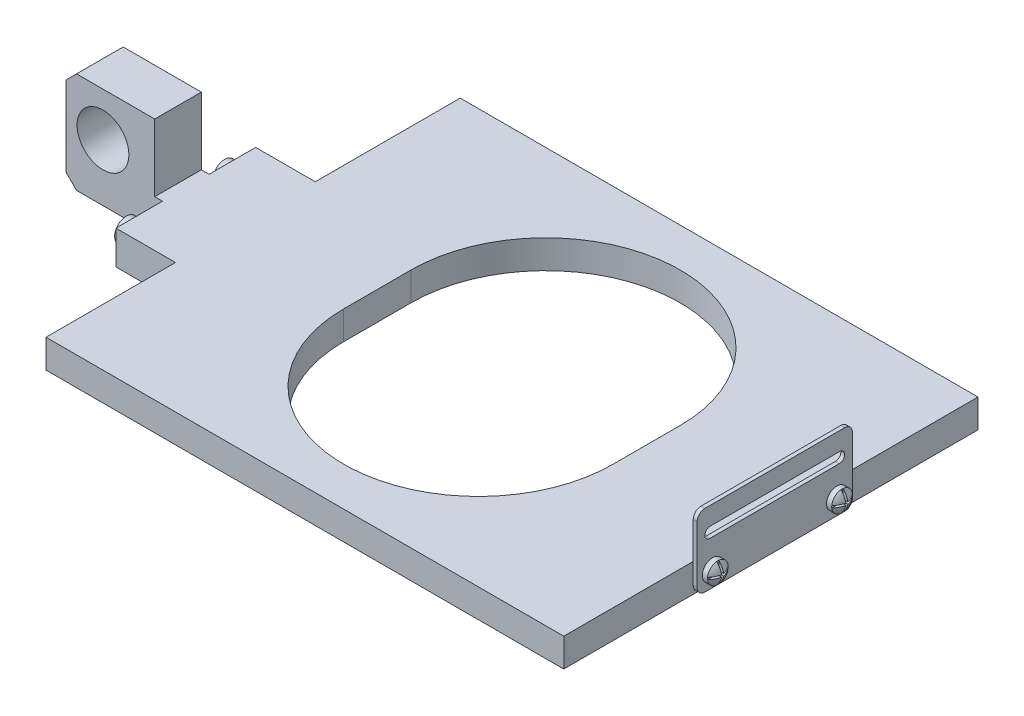
from build123d import *

# Parameters (mm, degrees)
EXTRUDE_1_DEPTH      = 50
EXTRUDE_1_DEPTH_BACK = 50
SKETCH_1_W           = 80
SKETCH_1_H           = 5.5
EXTRUDE_2_DEPTH      = 40
EXTRUDE_2_DEPTH_BACK = 40
SKETCH_2_R           = 5
CUT_EXTRUDE_1_DEPTH  = 45
EXTRUDE_3_DEPTH      = 0.75
CUT_EXTRUDE_2_DEPTH  = 1
CUT_EXTRUDE_3_DEPTH  = 1
CUT_EXTRUDE_4_DEPTH  = 50
SKETCH_10_R          = 2.25
EXTRUDE_4_DEPTH      = 2
SKETCH_11_R          = 2.25
EXTRUDE_5_DEPTH      = 2
CUT_EXTRUDE_5_DEPTH  = 1
CUT_EXTRUDE_6_DEPTH  = 1


with BuildPart() as part:
    # 草图1 → 凸台-拉伸1 (new, two sides: drawn at the far end of the back side and taken through both)
    with BuildSketch(Plane(origin=(0, 0, 0), x_dir=(0, 0, -1), z_dir=(1, 0, 0)).offset(-EXTRUDE_1_DEPTH_BACK)):
        with Locations((0, 4.75)):
            Rectangle(SKETCH_1_W, SKETCH_1_H)
    extrude(amount=EXTRUDE_1_DEPTH + EXTRUDE_1_DEPTH_BACK)

    # 草图2 → 凸台-拉伸2 (add, two sides: drawn at the far end of the back side and taken through both)
    with BuildSketch(Plane.XY.offset(-EXTRUDE_2_DEPTH_BACK)):
        Polygon((-80.1, 18.5), (-80.1, 3), (-78.1, 1), (-50, 1), (-50, 7.5), (-63, 7.5), (-63, 20.5), (-78.1, 20.5), align=None)
        with Locations((-73, 12)):
            Circle(SKETCH_2_R, mode=Mode.SUBTRACT)
    extrude(amount=EXTRUDE_2_DEPTH + EXTRUDE_2_DEPTH_BACK)

    # 草图3 → 切除-拉伸1 (cut)
    with BuildSketch(Plane(origin=(0, 0, 0), x_dir=(-1, 0, 0), z_dir=(0, 1, 0))):
        Polygon((84.5, -50), (84.5, 50), (50, 50), (50, 15), (61.5, 15), (61.5, 6), (82, 6), (82, -3), (61.5, -3), (61.5, -12), (50, -12), (50, -50), align=None)
    extrude(amount=CUT_EXTRUDE_1_DEPTH, mode=Mode.SUBTRACT)

    # 草图4 → 凸台-拉伸3 (add)
    with BuildSketch(Plane(origin=(50, 0, 0), x_dir=(0, 0, -1), z_dir=(1, 0, 0))):
        with BuildLine():
            Line((-15, 14.5), (-15, 3.5))
            ThreePointArc((-15, 3.5), (-14.560660172, 2.439339828), (-13.5, 2))
            Line((-13.5, 2), (13.5, 2))
            ThreePointArc((13.5, 2), (14.560660172, 2.439339828), (15, 3.5))
            Line((15, 3.5), (15, 14.5))
            ThreePointArc((15, 14.5), (14.560660172, 15.560660172), (13.5, 16))
            Line((13.5, 16), (-13.5, 16))
            ThreePointArc((-13.5, 16), (-14.560660172, 15.560660172), (-15, 14.5))
        make_face()
        with BuildLine():
            Line((-12.5, 10.5), (12.5, 10.5))
            ThreePointArc((12.5, 10.5), (13.5, 11.5), (12.5, 12.5))
            Line((12.5, 12.5), (-12.5, 12.5))
            ThreePointArc((-12.5, 12.5), (-13.5, 11.5), (-12.5, 10.5))
        make_face(mode=Mode.SUBTRACT)
    extrude(amount=EXTRUDE_3_DEPTH)

    # 草图5 → 旋转1 (revolve)
    with BuildSketch(Plane.XY.offset(12), mode=Mode.PRIVATE) as revolve_1_sk:
        with BuildLine():
            Line((50.75, 5), (50.75, 7))
            Line((50.75, 7), (51.75, 7))
            ThreePointArc((51.75, 7), (52.381148113, 6.065574057), (52.75, 5))
            Line((52.75, 5), (50.75, 5))
        make_face()
    revolve(revolve_1_sk.sketch.rotate(Axis((52.75, 5, 12), (-1, 0, 0)), 270), axis=Axis((52.75, 5, 12), (-1, 0, 0)))

    # 草图6 → 旋转2 (revolve)
    with BuildSketch(Plane.XY.offset(-12), mode=Mode.PRIVATE) as revolve_2_sk:
        with BuildLine():
            Line((50.75, 5), (50.75, 7))
            Line((50.75, 7), (51.75, 7))
            ThreePointArc((51.75, 7), (52.381148113, 6.065574057), (52.75, 5))
            Line((52.75, 5), (50.75, 5))
        make_face()
    revolve(revolve_2_sk.sketch.rotate(Axis((52.75, 5, -12), (-1, 0, 0)), 270), axis=Axis((52.75, 5, -12), (-1, 0, 0)))

    # 草图7 → 切除-拉伸2 (cut)
    with BuildSketch(Plane(origin=(52.75, 0, 0), x_dir=(0, 0, -1), z_dir=(1, 0, 0))):
        with BuildLine():
            Line((10.010025126, 4.8), (11.8, 4.8))
            Line((11.8, 4.8), (11.8, 3.010025126))
            ThreePointArc((11.8, 3.010025126), (12, 3), (12.2, 3.010025126))
            Line((12.2, 3.010025126), (12.2, 4.8))
            Line((12.2, 4.8), (13.989974874, 4.8))
            ThreePointArc((13.989974874, 4.8), (14, 5), (13.989974874, 5.2))
            Line((13.989974874, 5.2), (12.2, 5.2))
            Line((12.2, 5.2), (12.2, 6.989974874))
            ThreePointArc((12.2, 6.989974874), (12, 7), (11.8, 6.989974874))
            Line((11.8, 6.989974874), (11.8, 5.2))
            Line((11.8, 5.2), (10.010025126, 5.2))
            ThreePointArc((10.010025126, 5.2), (10, 5), (10.010025126, 4.8))
        make_face()
    extrude(amount=-CUT_EXTRUDE_2_DEPTH, mode=Mode.SUBTRACT)

    # 草图8 → 切除-拉伸3 (cut)
    with BuildSketch(Plane(origin=(52.75, 0, 0), x_dir=(0, 0, -1), z_dir=(1, 0, 0))):
        with BuildLine():
            Line((-13.989974874, 4.8), (-12.2, 4.8))
            Line((-12.2, 4.8), (-12.2, 3.010025126))
            ThreePointArc((-12.2, 3.010025126), (-12, 3), (-11.8, 3.010025126))
            Line((-11.8, 3.010025126), (-11.8, 4.8))
            Line((-11.8, 4.8), (-10.010025126, 4.8))
            ThreePointArc((-10.010025126, 4.8), (-10, 5), (-10.010025126, 5.2))
            Line((-10.010025126, 5.2), (-11.8, 5.2))
            Line((-11.8, 5.2), (-11.8, 6.989974874))
            ThreePointArc((-11.8, 6.989974874), (-12, 7), (-12.2, 6.989974874))
            Line((-12.2, 6.989974874), (-12.2, 5.2))
            Line((-12.2, 5.2), (-13.989974874, 5.2))
            ThreePointArc((-13.989974874, 5.2), (-14, 5), (-13.989974874, 4.8))
        make_face()
    extrude(amount=-CUT_EXTRUDE_3_DEPTH, mode=Mode.SUBTRACT)

    # 草图9 → 切除-拉伸4 (cut)
    with BuildSketch(Plane(origin=(0, 0, 0), x_dir=(-1, 0, 0), z_dir=(0, 1, 0))):
        with BuildLine():
            Line((-26, 6.5), (-26, -6.5))
            ThreePointArc((-26, -6.5), (0, -32.5), (26, -6.5))
            Line((26, -6.5), (26, 6.5))
            ThreePointArc((26, 6.5), (0, 32.5), (-26, 6.5))
        make_face()
    extrude(amount=CUT_EXTRUDE_4_DEPTH, mode=Mode.SUBTRACT)

    # 草图10 → 凸台-拉伸4 (add)
    with BuildSketch(Plane.ZY.offset(61.5)):
        with Locations((-8, 4.25)):
            Circle(SKETCH_10_R)
    extrude(amount=EXTRUDE_4_DEPTH)

    # 草图11 → 凸台-拉伸5 (add)
    with BuildSketch(Plane.ZY.offset(61.5)):
        with Locations((11, 4.25)):
            Circle(SKETCH_11_R)
    extrude(amount=EXTRUDE_5_DEPTH)

    # 草图12 → 切除-拉伸5 (cut)
    with BuildSketch(Plane.ZY.offset(63.5)):
        Polygon((-7.422649731, 3.25), (-6.845299462, 4.25), (-7.422649731, 5.25), (-8.577350269, 5.25), (-9.154700538, 4.25), (-8.577350269, 3.25), align=None)
    extrude(amount=-CUT_EXTRUDE_5_DEPTH, mode=Mode.SUBTRACT)

    # 草图13 → 切除-拉伸6 (cut)
    with BuildSketch(Plane.ZY.offset(63.5)):
        Polygon((11.577350269, 3.25), (12.154700538, 4.25), (11.577350269, 5.25), (10.422649731, 5.25), (9.845299462, 4.25), (10.422649731, 3.25), align=None)
    extrude(amount=-CUT_EXTRUDE_6_DEPTH, mode=Mode.SUBTRACT)


solid = part.part
